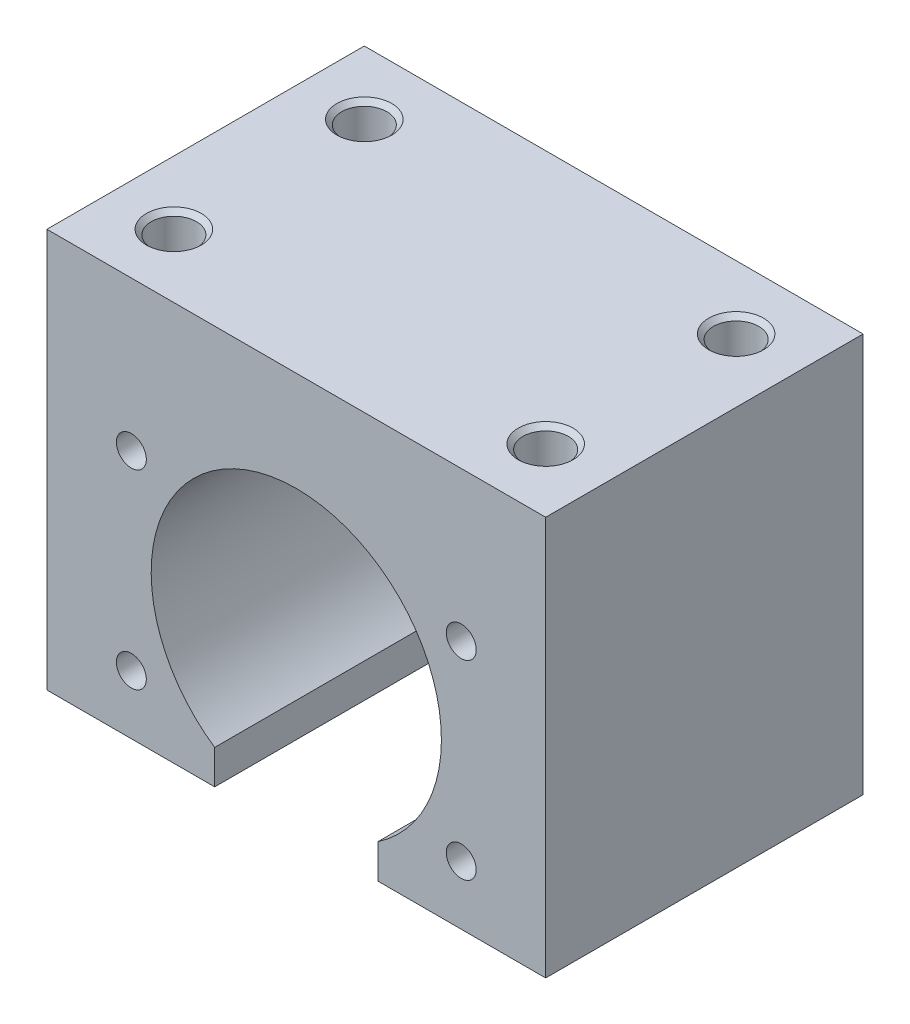
from build123d import *

# Parameters (mm, degrees)
EXTRUDE_1_DEPTH              = 17.5
HOLE_WIZARD_M4_1_D           = 3.3
HOLE_WIZARD_M4_1_DEPTH       = 9.5
HOLE_WIZARD_M4_1_TIP         = 0.991420021
HOLE_WIZARD_M6_1_D           = 5
HOLE_WIZARD_M6_1_DEPTH       = 12
HOLE_WIZARD_M6_1_CSINK_D     = 6.05
HOLE_WIZARD_M6_1_CSINK_ANGLE = 90
HOLE_WIZARD_M6_1_TIP         = 1.502151548


with BuildPart() as part:
    # 草图1 → 凸台-拉伸1 (new, symmetric)
    with BuildSketch(Plane.XY):
        with BuildLine():
            Line((-27.5, 27), (27.5, 27))
            Line((27.5, 27), (27.5, -17))
            Line((27.5, -17), (9, -17))
            Line((9, -17), (9, -13.228756555))
            ThreePointArc((9, -13.228756555), (0, 16), (-9, -13.228756555))
            Line((-9, -13.228756555), (-9, -17))
            Line((-9, -17), (-27.5, -17))
            Line((-27.5, -17), (-27.5, 27))
        make_face()
    extrude(amount=EXTRUDE_1_DEPTH, both=True)

    # M4 螺纹孔1
    with Locations(Plane.XY.offset(17.5)):
        with Locations((18.186533479, 10.5), (18.186533479, -10.5), (-18.186533479, -10.5), (-18.186533479, 10.5)):
            Hole(HOLE_WIZARD_M4_1_D / 2, depth=HOLE_WIZARD_M4_1_DEPTH)
            with Locations((0, 0, -(HOLE_WIZARD_M4_1_DEPTH + HOLE_WIZARD_M4_1_TIP / 2))):  # 118° drill point
                Cone(0, HOLE_WIZARD_M4_1_D / 2, HOLE_WIZARD_M4_1_TIP, mode=Mode.SUBTRACT)

    # M6 螺纹孔1
    with Locations(Plane(origin=(-20.5, 27, 10.5), x_dir=(0, 0, 1), z_dir=(0, 1, 0))):
        with Locations((0, 0), (-21, 0), (-21, 41), (0, 41)):
            CounterSinkHole(HOLE_WIZARD_M6_1_D / 2, HOLE_WIZARD_M6_1_CSINK_D / 2, depth=HOLE_WIZARD_M6_1_DEPTH, counter_sink_angle=HOLE_WIZARD_M6_1_CSINK_ANGLE)
            with Locations((0, 0, -(HOLE_WIZARD_M6_1_DEPTH + HOLE_WIZARD_M6_1_TIP / 2))):  # 118° drill point
                Cone(0, HOLE_WIZARD_M6_1_D / 2, HOLE_WIZARD_M6_1_TIP, mode=Mode.SUBTRACT)


solid = part.part
